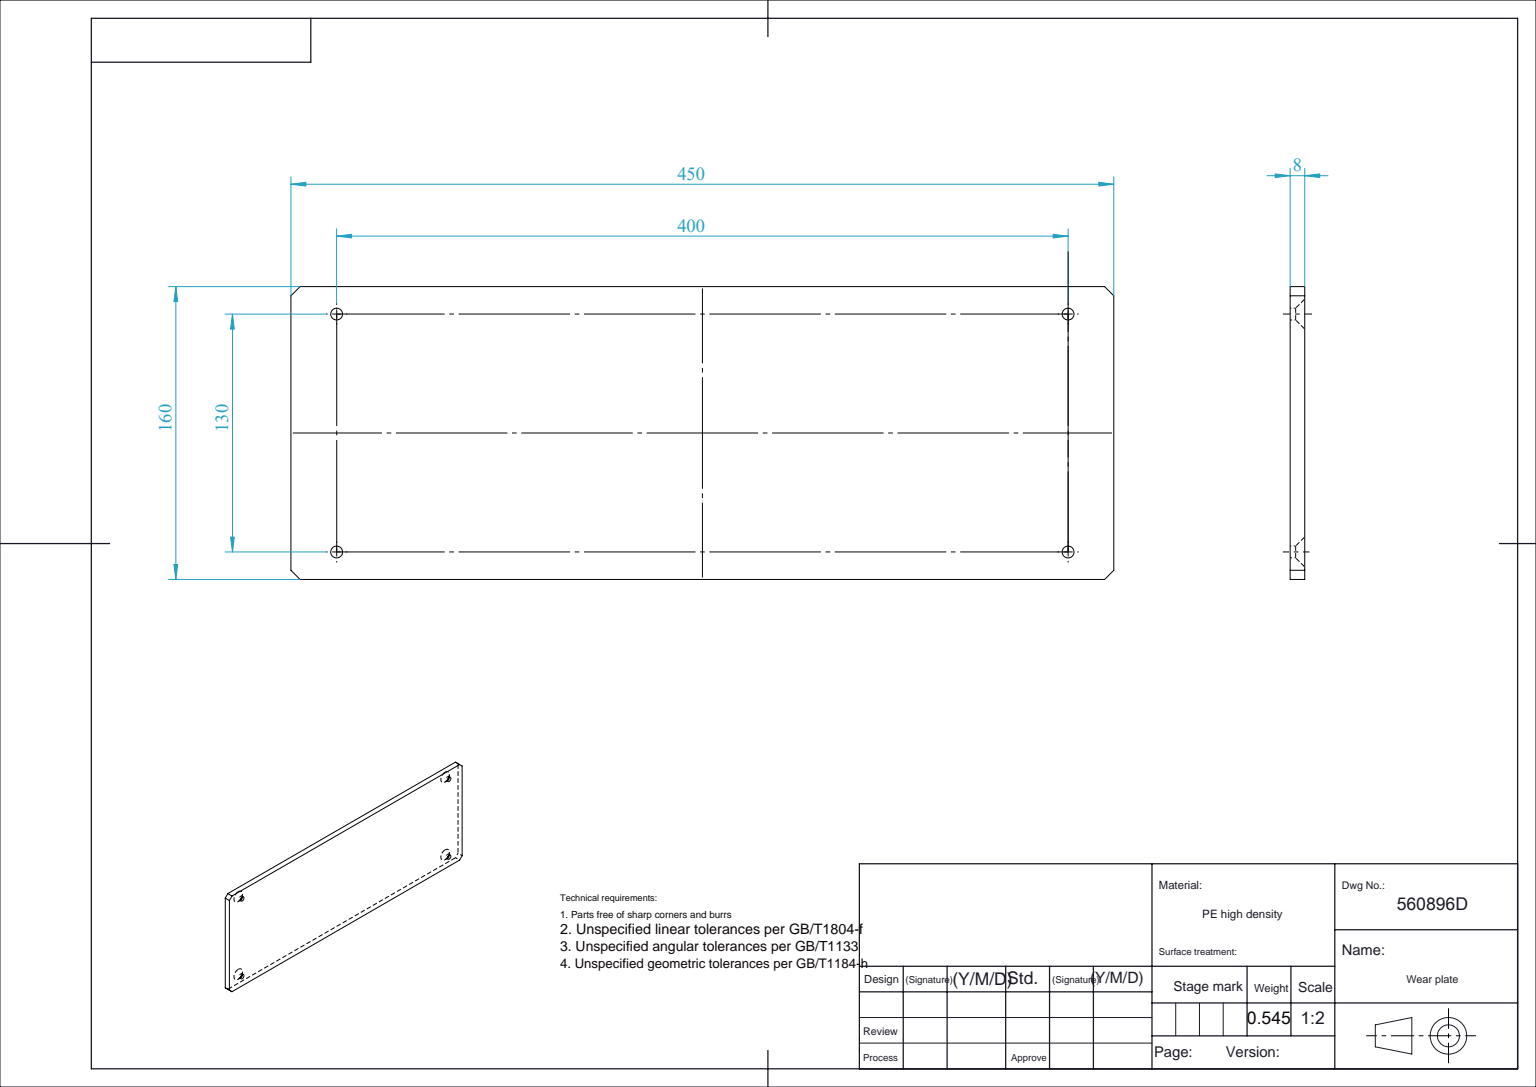
SolidWorks part; units mm, degrees
material "HDPE"
ref_plane "Front Plane" through (0, 0, 0) normal (0, 0, 1) x (1, 0, 0)
ref_plane "Top Plane" through (0, 0, 0) normal (0, 1, 0) x (1, 0, 0)
ref_plane "Right Plane" through (0, 0, 0) normal (1, 0, 0) x (0, 0, -1)
sketch "Sketch1" plane through (0, 0, 0) normal (0, 1, 0) x (1, 0, 0)
  line L1 (-225, 80) -> (225, 80)
  line L2 (-225, 80) -> (-225, -80)
  line L3 (-225, -80) -> (225, -80)
  line L4 (225, 80) -> (225, -80)
  line L5 (-225, 80) -> (225, -80) construction
  line L6 (-225, -80) -> (225, 80) construction
  point P0 (0, 0)
  dimension "D1" = 450
  dimension "D2" = 160
extrude "Boss-Extrude1" add sketch "Sketch1" along normal blind 8 contours L2 L1 L4 L3
sketch "Sketch15" plane through (0, 0, 0) normal (0, -1, 0) x (1, 0, 0)
  line L0 (-225, 80) -> (225, 80) construction
  line L1 (-225, -80) -> (-225, 80) construction
  circle A0 centre (-200, 65) radius 3.25
  circle A1 centre (-200, -65) radius 3.25
  circle A2 centre (200, 65) radius 3.25
  circle A3 centre (200, -65) radius 3.25
  dimension "D5" = 6.5
  dimension "D1" = 15
  dimension "D2" = 130
  dimension "D3" = 400
  dimension "D4" = 25
extrude "Cut-Extrude5" cut sketch "Sketch15" against normal blind 8
sketch "Sketch16" plane through (0, 0, 0) normal (0, -1, 0) x (1, 0, 0)
  circle A0 centre (-200, 65) radius 8.25
  circle A1 centre (-200, -65) radius 8.25
  circle A2 centre (200, 65) radius 8.25
  circle A3 centre (200, -65) radius 8.25
  dimension "D1" = 16.5
extrude "Cut-Extrude6" cut sketch "Sketch16" against normal blind 5 draft 45
chamfer "Chamfer1" distance 5 angle 45 4 edges at (225, 4, -80) (225, 4, 80) (-225, 4, -80) (-225, 4, 80)
